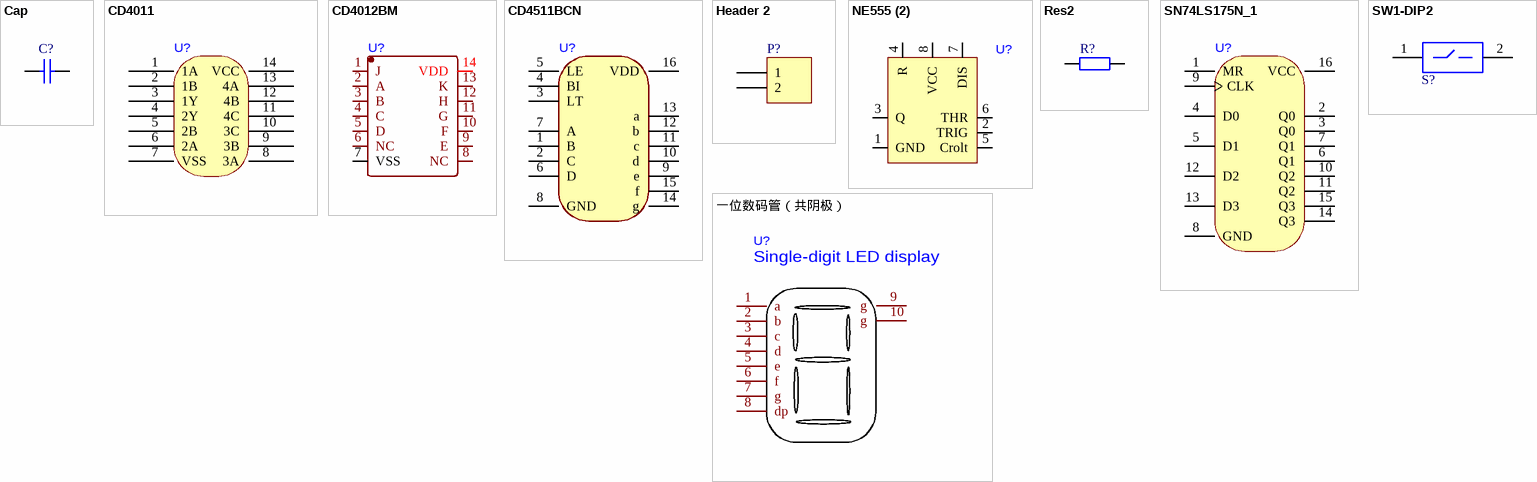
[diagram p0: symbols Cap to 一位数码管（共阴极）]
# Altium schematic symbol library MISC80628-24.SCHLIB: 10 symbols
Pins are listed as number, name and electrical type; pins without a type are passive.


## Cap
designator C?
Capacitor
footprint RAD-0.3 (Radial Cap, Thru-Hole; 2 Leads; 0.3 in Pin Spacing)
simulation model CAP (Capacitor)
signal-integrity model Cap
pins: 1, 2

## CD4011
designator U?
footprint CD4011
pins: 1 1A, 2 1B, 3 1Y, 4 2Y, 5 2B, 6 2A, 7 VSS, 8 3A, 9 3B, 10 3C, 11 4C, 12 4B, 13 4A, 14 VCC

## CD4012BM
designator U?
footprint DIP14 (Footprint not found)
pins: 1 J, 2 A, 3 B, 4 C, 5 D, 6 NC, 7 VSS, 8 NC, 9 E, 10 F, 11 G, 12 H, 13 K, 14 VDD

## CD4511BCN
designator U?
footprint CD4511BCN
pins: 1 B, 2 C, 3 LT, 4 BI, 5 LE, 6 D, 7 A, 8 GND, 9 e, 10 d, 11 c, 12 b, 13 a, 14 g, 15 f, 16 VDD

## Header 2
designator P?
Header, 2-Pin
footprint HDR1X2 (Connector; Header; 2 Position)
signal-integrity model Connector
pins: 1, 2

## NE555 (2)
designator U?
footprint DIP-8-NE555
pins: 1 GND, 2 TRIG, 3 Q, 4 R, 5 Crolt, 6 THR, 7 DIS, 8 VCC

## Res2
designator R?
Resistor
footprint AXIAL-0.4 (Axial Device, Thru-Hole; 2 Leads; 0.4 in Pin Spacing)
simulation model RESISTOR (Resistor)
signal-integrity model Res
pins: 1, 2

## SN74LS175N_1
designator U?
footprint 0
footprint N016
pins: 1 MR, 2 Q0, 3 Q0, 4 D0, 5 D1, 6 Q1, 7 Q1, 8 GND, 9 CLK, 10 Q2, 11 Q2, 12 D2, 13 D3, 14 Q3, 15 Q3, 16 VCC

## SW1-DIP2
designator S?
footprint DIP-1P (4.1*9.9*7mm)
footprint DIP-1P_R (4.1*9.9*7mm)
pins: 1 A1, 2

## 一位数码管（共阴极）
designator U?
footprint PCBComponent_1 (Footprint not found)
pins: 1 a, 2 b, 3 c, 4 d, 5 e, 6 f, 7 g, 8 dp, 9 g, 10 g